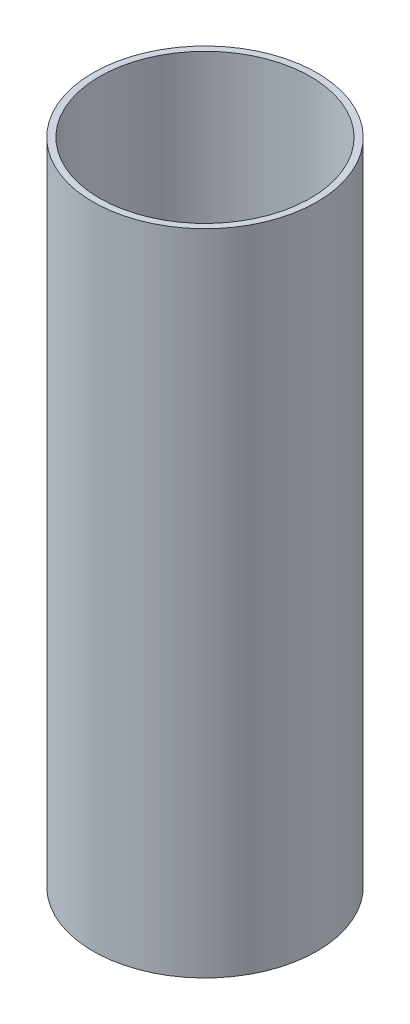
from build123d import *

# Parameters (mm, degrees)
SKETCH1_R           = 3.45
SKETCH1_R_2         = 3.25
EXTRUDE_THIN1_DEPTH = 20


with BuildPart() as part:
    # Sketch1 → Extrude-Thin1 (new body)
    with BuildSketch(Plane(origin=(0, 0, 0), x_dir=(1, 0, 0), z_dir=(0, 1, 0))):
        Circle(SKETCH1_R)
        Circle(SKETCH1_R_2, mode=Mode.SUBTRACT)
    extrude(amount=EXTRUDE_THIN1_DEPTH)


solid = part.part
